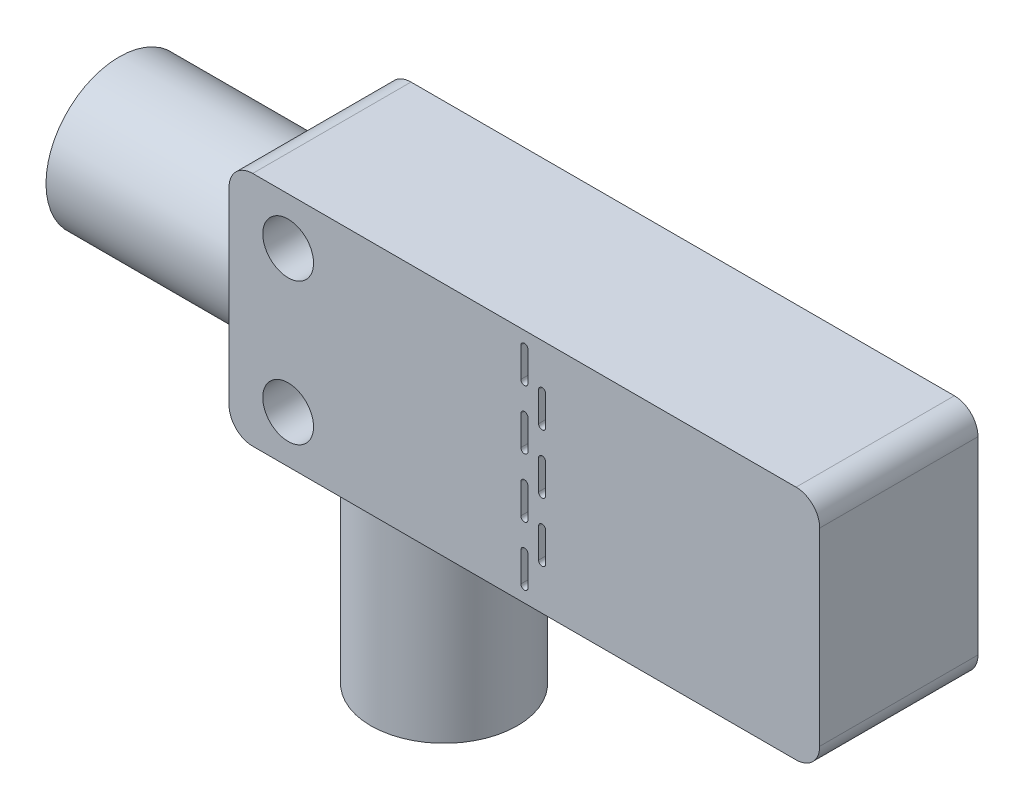
from build123d import *

# Parameters (mm, degrees)
SKETCH_1_W                  = 50
SKETCH_1_H                  = 20
EXTRUDE_1_DEPTH             = 13.4
SKETCH_2_R                  = 6.2
EXTRUDE_2_DEPTH             = 16
SKETCH_3_R                  = 6.2
EXTRUDE_3_DEPTH             = 16
HOLE_WIZARD_6_0_6_1_D       = 6
HOLE_WIZARD_6_0_6_1_DEPTH   = 30
HOLE_WIZARD_6_0_6_1_TIP     = 1.802581857
HOLE_WIZARD_6_0_6_2_D       = 6
HOLE_WIZARD_6_0_6_2_DEPTH   = 30
HOLE_WIZARD_6_0_6_2_TIP     = 1.802581857
HOLE_WIZARD_4_3_4_3_1_D     = 4.3
HOLE_WIZARD_4_3_4_3_1_DEPTH = 30
HOLE_WIZARD_4_3_4_3_1_TIP   = 1.291850331
FILLET_1_R                  = 2
CUT_EXTRUDE_1_REACH         = 52.364
PATTERN_LINEAR_1_COUNT      = 4
PATTERN_LINEAR_1_PITCH      = 5
CUT_EXTRUDE_2_REACH         = 52.364
PATTERN_LINEAR_2_COUNT      = 3
PATTERN_LINEAR_2_PITCH      = 5


with BuildPart() as part:
    # 草图1 → 凸台-拉伸1 (new body)
    with BuildSketch(Plane.XY):
        Rectangle(SKETCH_1_W, SKETCH_1_H)
    extrude(amount=EXTRUDE_1_DEPTH)

    # 草图2 → 凸台-拉伸2 (add)
    with BuildSketch(Plane.XZ.offset(10)):
        with Locations(Location((-13.5, 6.7, 0), (0, 0, 90))):
            Circle(SKETCH_2_R)
    extrude(amount=EXTRUDE_2_DEPTH)

    # 草图3 → 凸台-拉伸3 (add)
    with BuildSketch(Plane.ZY.offset(25)):
        with Locations(Location((6.7, 0, 0), (0, 0, 180))):
            Circle(SKETCH_3_R)
    extrude(amount=EXTRUDE_3_DEPTH)

    # Ø6.0 (6) 直径孔1
    with Locations(Plane.ZY.offset(41)):
        with Locations((6.7, 0)):
            Hole(HOLE_WIZARD_6_0_6_1_D / 2, depth=HOLE_WIZARD_6_0_6_1_DEPTH)
            with Locations((0, 0, -(HOLE_WIZARD_6_0_6_1_DEPTH + HOLE_WIZARD_6_0_6_1_TIP / 2))):  # 118° drill point
                Cone(0, HOLE_WIZARD_6_0_6_1_D / 2, HOLE_WIZARD_6_0_6_1_TIP, mode=Mode.SUBTRACT)

    # Ø6.0 (6) 直径孔2
    with Locations(Plane.XZ.offset(26)):
        with Locations((-13.5, 6.7)):
            Hole(HOLE_WIZARD_6_0_6_2_D / 2, depth=HOLE_WIZARD_6_0_6_2_DEPTH)
            with Locations((0, 0, -(HOLE_WIZARD_6_0_6_2_DEPTH + HOLE_WIZARD_6_0_6_2_TIP / 2))):  # 118° drill point
                Cone(0, HOLE_WIZARD_6_0_6_2_D / 2, HOLE_WIZARD_6_0_6_2_TIP, mode=Mode.SUBTRACT)

    # Ø4.3 (4.3) 直径孔1
    with Locations(Plane.XY.offset(13.4)):
        with Locations((-20, 6), (-20, -6)):
            Hole(HOLE_WIZARD_4_3_4_3_1_D / 2, depth=HOLE_WIZARD_4_3_4_3_1_DEPTH)
            with Locations((0, 0, -(HOLE_WIZARD_4_3_4_3_1_DEPTH + HOLE_WIZARD_4_3_4_3_1_TIP / 2))):  # 118° drill point
                Cone(0, HOLE_WIZARD_4_3_4_3_1_D / 2, HOLE_WIZARD_4_3_4_3_1_TIP, mode=Mode.SUBTRACT)

    # 圆角1
    fillet_1_edges = [part.edges().sort_by_distance(p)[0] for p in [
        (25, -10, 6.7),
        (-25, -10, 6.7),
        (-25, 10, 6.7),
        (25, 10, 6.7),
    ]]
    fillet(fillet_1_edges, radius=FILLET_1_R)

    # 草图11 → 切除-拉伸1 (cut, up to next)
    with BuildSketch(Plane.XY.offset(13.4), mode=Mode.PRIVATE) as cut_extrude_1_sk1:
        with BuildLine():
            Line((0.3, 8.75), (0.3, 6.25))
            ThreePointArc((0.3, 6.25), (0, 5.95), (-0.3, 6.25))
            Line((-0.3, 6.25), (-0.3, 8.75))
            ThreePointArc((-0.3, 8.75), (0, 9.05), (0.3, 8.75))
        make_face()
    cut_extrude_1_tool1 = extrude(cut_extrude_1_sk1.sketch, amount=-CUT_EXTRUDE_1_REACH, mode=Mode.PRIVATE) & part.part
    cut_extrude_1 = cut_extrude_1_tool1.solids().sort_by_distance((0, 7.5, 13.4))[0]
    add(cut_extrude_1, mode=Mode.SUBTRACT)

    # 阵列(线性)1: 切除-拉伸1 ×4
    with Locations(*[(0, -i * PATTERN_LINEAR_1_PITCH, 0) for i in range(1, PATTERN_LINEAR_1_COUNT)]):
        add(cut_extrude_1, mode=Mode.SUBTRACT)

    # 草图12 → 切除-拉伸2 (cut, up to next)
    with BuildSketch(Plane.XY.offset(13.4), mode=Mode.PRIVATE) as cut_extrude_2_sk1:
        with BuildLine():
            Line((1.8, 6.25), (1.8, 3.75))
            ThreePointArc((1.8, 3.75), (1.5, 3.45), (1.2, 3.75))
            Line((1.2, 3.75), (1.2, 6.25))
            ThreePointArc((1.2, 6.25), (1.5, 6.55), (1.8, 6.25))
        make_face()
    cut_extrude_2_tool1 = extrude(cut_extrude_2_sk1.sketch, amount=-CUT_EXTRUDE_2_REACH, mode=Mode.PRIVATE) & part.part
    cut_extrude_2 = cut_extrude_2_tool1.solids().sort_by_distance((1.5, 5, 13.4))[0]
    add(cut_extrude_2, mode=Mode.SUBTRACT)

    # 阵列(线性)2: 切除-拉伸2 ×3
    with Locations(*[(0, -i * PATTERN_LINEAR_2_PITCH, 0) for i in range(1, PATTERN_LINEAR_2_COUNT)]):
        add(cut_extrude_2, mode=Mode.SUBTRACT)


solid = part.part
